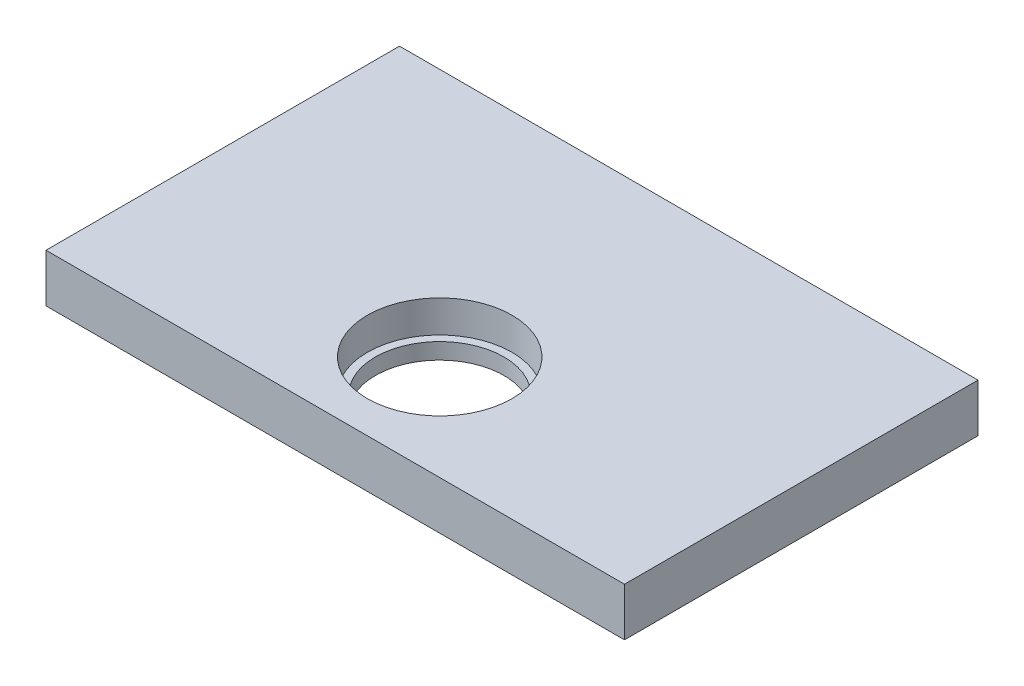
SolidWorks part; units mm, degrees
ref_plane "前视基准面" through (0, 0, 0) normal (0, 0, 1) x (1, 0, 0)
ref_plane "上视基准面" through (0, 0, 0) normal (0, 1, 0) x (1, 0, 0)
ref_plane "右视基准面" through (0, 0, 0) normal (1, 0, 0) x (0, 0, -1)
sketch "草图1" plane through (0, 0, 0) normal (0, 1, 0) x (1, 0, 0)
  line L1 (-180, -110) -> (180, -110)
  line L2 (-180, -110) -> (-180, 110)
  line L3 (-180, 110) -> (180, 110)
  line L4 (180, -110) -> (180, 110)
  line L5 (-180, -110) -> (180, 110) construction
  line L6 (-180, 110) -> (180, -110) construction
  point P0 (0, 0)
  dimension "D1" = 360
  dimension "D2" = 220
extrude "凸台-拉伸1" add sketch "草图1" along normal blind 30
sketch "草图2" plane through (0, 30, 0) normal (0, 1, 0) x (1, 0, 0)
  line L0 (180, -110) -> (180, 110) construction
  line L1 (180, 110) -> (-180, 110) construction
  circle A0 centre (0, -45) radius 40
  dimension "D1" = 80
  dimension "D2" = 180
  dimension "D3" = 155
extrude "切除-拉伸1" cut sketch "草图2" against normal through all
sketch "草图3" plane through (0, 30, 0) normal (0, -1, 0) x (1, 0, 0)
  line L0 (180, 110) -> (180, -110) construction
  line L1 (-180, 110) -> (180, 110) construction
  circle A0 centre (0, 45) radius 45
  dimension "D1" = 90
  dimension "D2" = 180
  dimension "D3" = 65
extrude "切除-拉伸2" cut sketch "草图3" along normal blind 20
